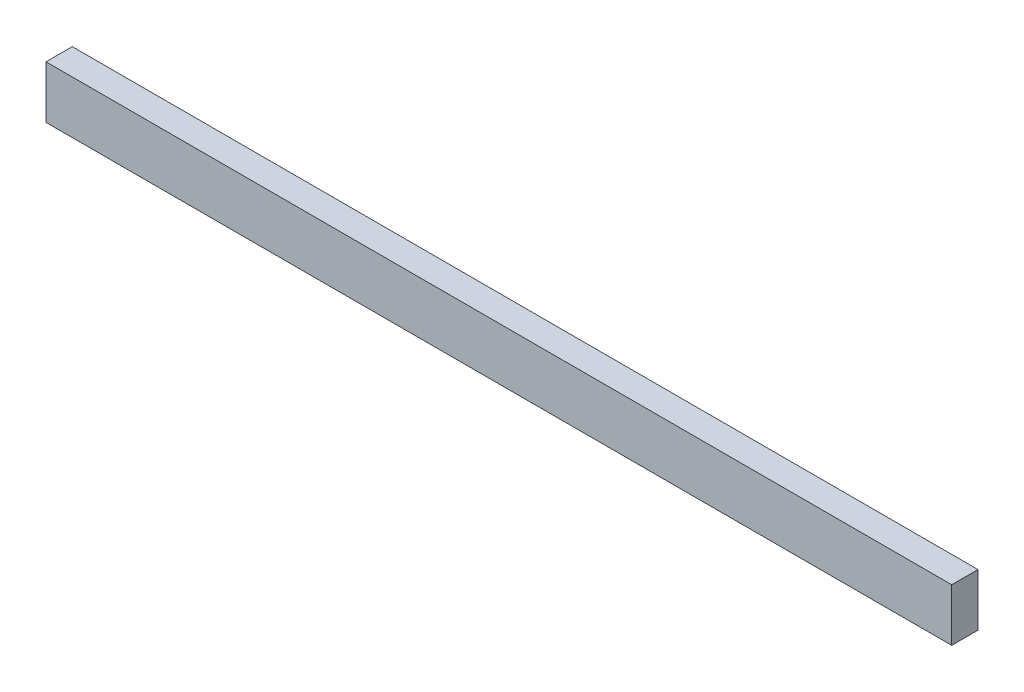
from build123d import *

# Parameters (mm, degrees)
SKETCH1_W           = 345
SKETCH1_H           = 20
BOSS_EXTRUDE1_DEPTH = 10


with BuildPart() as part:
    # Sketch1 → Boss-Extrude1 (new body)
    with BuildSketch(Plane.XY):
        Rectangle(SKETCH1_W, SKETCH1_H)
    extrude(amount=BOSS_EXTRUDE1_DEPTH)


solid = part.part
